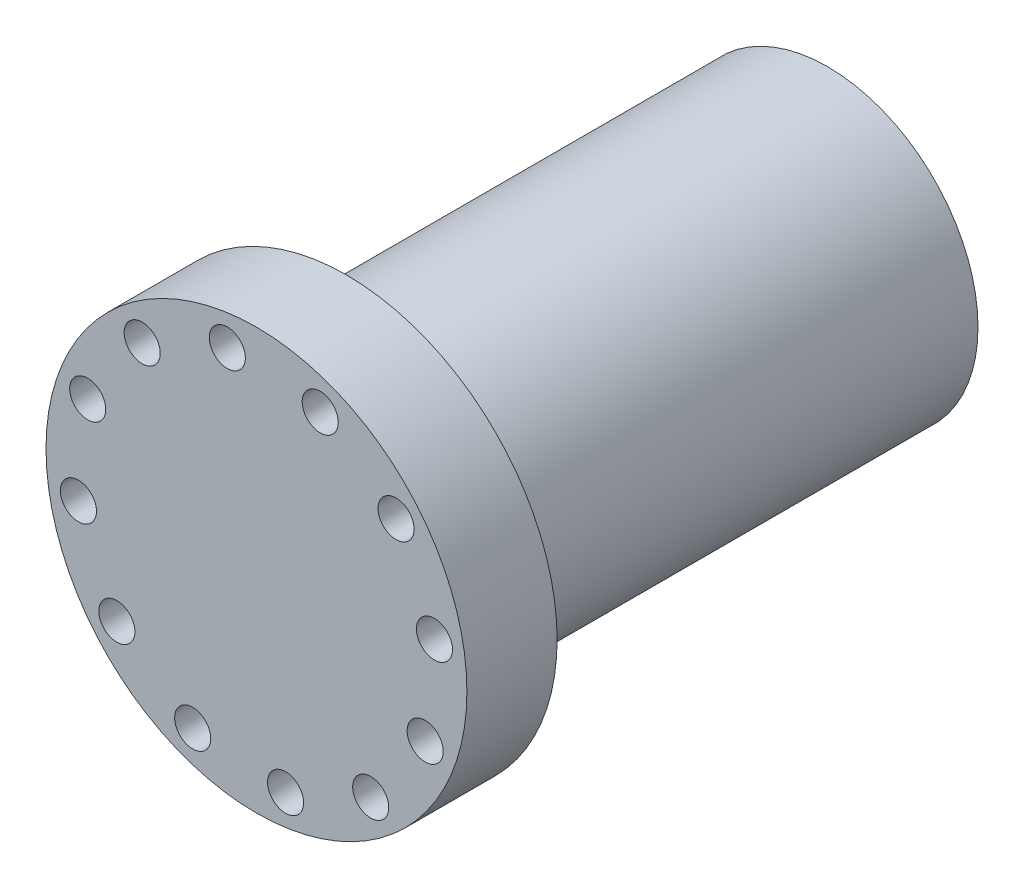
from build123d import *

# Parameters (mm, degrees)
SKETCH1_R               = 17.5
BOSS_EXTRUDE1_DEPTH     = 7.5
SKETCH2_R               = 12.5
BOSS_EXTRUDE2_DEPTH     = 40
CUT_EXTRUDE1_DEPTH      = 109.253175473
CUT_EXTRUDE1_DEPTH_BACK = 109.253175473
SKETCH3_R               = 1.5


with BuildPart() as part:
    # Sketch1 → Boss-Extrude1 (new body)
    with BuildSketch(Plane.XY):
        with Locations((-70, 25)):
            Circle(SKETCH1_R)
    extrude(amount=BOSS_EXTRUDE1_DEPTH)

    # Sketch2 → Boss-Extrude2 (add)
    with BuildSketch(Plane(origin=(0, 0, 0), x_dir=(-1, 0, 0), z_dir=(0, 0, -1))):
        with Locations((70, 25)):
            Circle(SKETCH2_R)
    extrude(amount=BOSS_EXTRUDE2_DEPTH)

    # Sketch3 → Cut-Extrude1 (cut, two sides: drawn at the far end of the back side and taken through both)
    with BuildSketch(Plane.XY.offset(7.5).offset(-CUT_EXTRUDE1_DEPTH_BACK)):
        with Locations((-81.608310906, 15.50015169)):
            Circle(SKETCH3_R)
        with Locations((-84.803016294, 22.577045484)):
            Circle(SKETCH3_R)
        with Locations((-84.031265422, 30.303167984)):
            Circle(SKETCH3_R)
        with Locations((-79.49984831, 36.608310906)):
            Circle(SKETCH3_R)
        with Locations((-72.422954516, 39.803016294)):
            Circle(SKETCH3_R)
        with Locations((-64.696832016, 39.031265422)):
            Circle(SKETCH3_R)
        with Locations((-58.391689094, 34.49984831)):
            Circle(SKETCH3_R)
        with Locations((-55.196983706, 27.422954516)):
            Circle(SKETCH3_R)
        with Locations((-55.968734578, 19.696832016)):
            Circle(SKETCH3_R)
        with Locations((-60.50015169, 13.391689094)):
            Circle(SKETCH3_R)
        with Locations((-67.577045484, 10.196983706)):
            Circle(SKETCH3_R)
        with Locations((-75.303167984, 10.968734578)):
            Circle(SKETCH3_R)
    extrude(amount=CUT_EXTRUDE1_DEPTH + CUT_EXTRUDE1_DEPTH_BACK, mode=Mode.SUBTRACT)


solid = part.part
